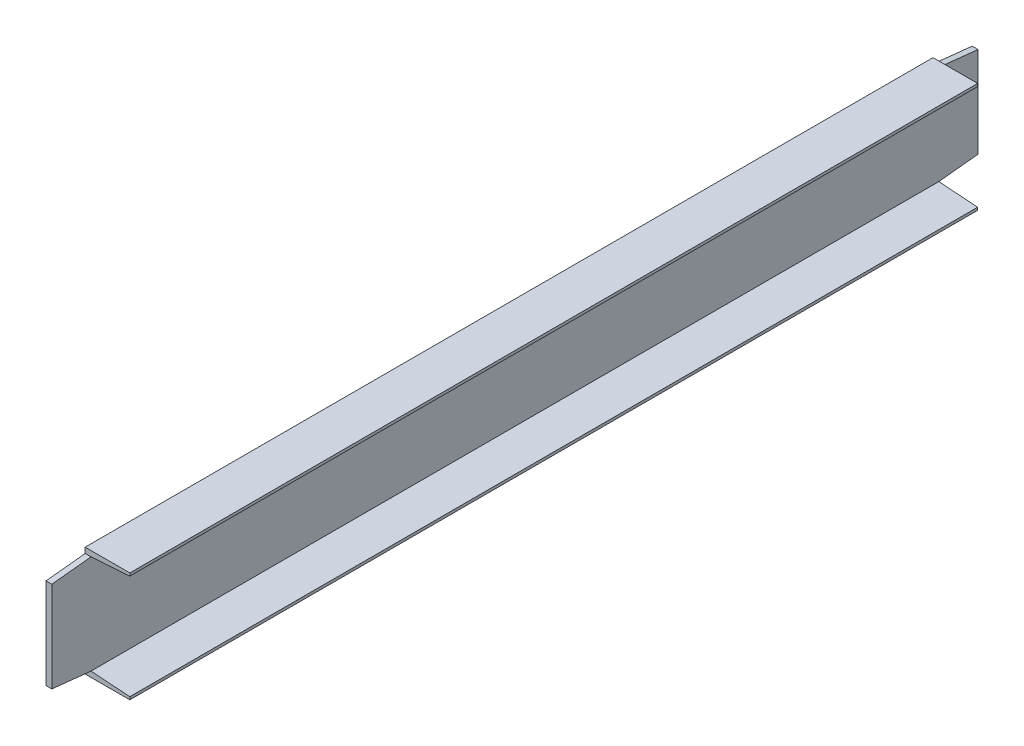
from build123d import *

# Parameters (mm, degrees)
EXTRUDE_1_DEPTH     = 674
CUT_EXTRUDE_1_DEPTH = 696.773670097


with BuildPart() as part:
    # 草图1 → 凸台-拉伸1 (new, symmetric)
    with BuildSketch(Plane.XY):
        Polygon((0, 0), (65, 0), (65, 4), (8.5, 8), (8.5, 152), (65, 156), (65, 160), (0, 160), align=None)
    extrude(amount=EXTRUDE_1_DEPTH, both=True)

    # 草图4 → 切除-拉伸1 (cut, through all)
    with BuildSketch(Plane.ZY):
        Polygon((-674, 160), (-617, 160), (-617, 152), (-674, 146), align=None)
        Polygon((674, 146), (674, 160), (617, 160), (617, 152), align=None)
        Polygon((674, 0), (617, 0), (617, 8), (674, 14), align=None)
        Polygon((-674, 14), (-674, 0), (-617, 0), (-617, 8), align=None)
    extrude(amount=-CUT_EXTRUDE_1_DEPTH, mode=Mode.SUBTRACT)


solid = part.part
